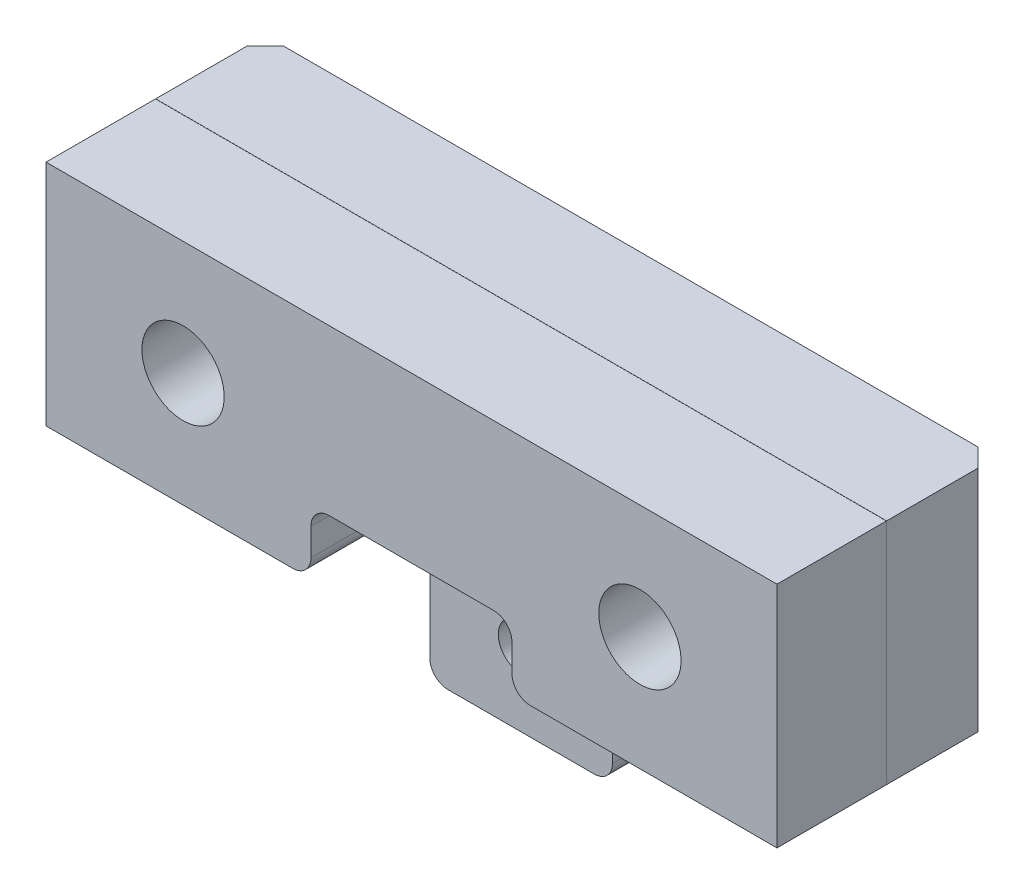
from build123d import *

# Parameters (mm, degrees)
SKETCH1_W                = 80
SKETCH1_H                = 24
BOSS_EXTRUDE1_DEPTH      = 20
CHAMFER1_SIZE            = 2
SKETCH9_W                = 20
SKETCH9_H                = 15
CUT_EXTRUDE1_DEPTH       = 12
M6_TAPPED_HOLE1_D        = 5
M6_TAPPED_HOLE1_DEPTH    = 15
M6_TAPPED_HOLE1_TIP      = 1.502151548
M8_CLEARANCE_HOLE1_D     = 9
M8_CLEARANCE_HOLE1_DEPTH = 30
M8_CLEARANCE_HOLE1_TIP   = 2.703872786
SKETCH16_W               = 30
SKETCH16_H               = 15
CUT_EXTRUDE2_DEPTH       = 86.883642214
FILLET1_R                = 5
FILLET2_R                = 2
SKETCH17_W               = 22
SKETCH17_H               = 7
CUT_EXTRUDE3_DEPTH       = 12
SKETCH18_W               = 80
SKETCH18_H               = 0.02
CUT_EXTRUDE4_DEPTH       = 88.183714076
FILLET3_R                = 2


with BuildPart() as part:
    # Sketch1 → Boss-Extrude1 (new, symmetric)
    with BuildSketch(Plane(origin=(0, 0, 0), x_dir=(1, 0, 0), z_dir=(0, 1, 0))):
        with Locations((40, 12)):
            Rectangle(SKETCH1_W, SKETCH1_H)
    extrude(amount=BOSS_EXTRUDE1_DEPTH, both=True)

    # Chamfer1
    chamfer1_edges = [part.edges().sort_by_distance(p)[0] for p in [
        (0, 0, -24),
        (80, 0, -24),
    ]]
    chamfer(chamfer1_edges, length=CHAMFER1_SIZE)

    # Sketch9 → Cut-Extrude1 (cut)
    with BuildSketch(Plane.XY):
        with Locations((40, -12.5)):
            Rectangle(SKETCH9_W, SKETCH9_H)
    extrude(amount=-CUT_EXTRUDE1_DEPTH, mode=Mode.SUBTRACT)

    # M6 Tapped Hole1
    with Locations(Plane(origin=(0, 0, -24), x_dir=(-1, 0, 0), z_dir=(0, 0, -1))):
        with Locations((-40, -12)):
            Hole(M6_TAPPED_HOLE1_D / 2, depth=M6_TAPPED_HOLE1_DEPTH)
            with Locations((0, 0, -(M6_TAPPED_HOLE1_DEPTH + M6_TAPPED_HOLE1_TIP / 2))):  # 118° drill point
                Cone(0, M6_TAPPED_HOLE1_D / 2, M6_TAPPED_HOLE1_TIP, mode=Mode.SUBTRACT)

    # M8 Clearance Hole1
    with Locations(Plane(origin=(0, 0, -24), x_dir=(-1, 0, 0), z_dir=(0, 0, -1))):
        with Locations((-65, 7.5), (-15, 7.5)):
            Hole(M8_CLEARANCE_HOLE1_D / 2, depth=M8_CLEARANCE_HOLE1_DEPTH)
            with Locations((0, 0, -(M8_CLEARANCE_HOLE1_DEPTH + M8_CLEARANCE_HOLE1_TIP / 2))):  # 118° drill point
                Cone(0, M8_CLEARANCE_HOLE1_D / 2, M8_CLEARANCE_HOLE1_TIP, mode=Mode.SUBTRACT)

    # Sketch16 → Cut-Extrude2 (cut, through all)
    with BuildSketch(Plane(origin=(0, 0, -24), x_dir=(-1, 0, 0), z_dir=(0, 0, -1))):
        with Locations((-65, -12.5)):
            Rectangle(SKETCH16_W, SKETCH16_H)
        with Locations((-15, -12.5)):
            Rectangle(SKETCH16_W, SKETCH16_H)
    extrude(amount=-CUT_EXTRUDE2_DEPTH, mode=Mode.SUBTRACT)

    # Fillet1
    fillet1_edges = [part.edges().sort_by_distance(p)[0] for p in [
        (50, -5, -18),
        (30, -5, -18),
    ]]
    fillet(fillet1_edges, radius=FILLET1_R)

    # Fillet2
    fillet2_edges = [part.edges().sort_by_distance(p)[0] for p in [
        (50, -20, -18),
        (30, -20, -18),
    ]]
    fillet(fillet2_edges, radius=FILLET2_R)

    # Sketch17 → Cut-Extrude3 (cut)
    with BuildSketch(Plane.XY):
        with Locations((40, -1.5)):
            Rectangle(SKETCH17_W, SKETCH17_H)
    extrude(amount=-CUT_EXTRUDE3_DEPTH, mode=Mode.SUBTRACT)

    # Sketch18 → Cut-Extrude4 (cut, through all)
    with BuildSketch(Plane.XZ.offset(5)):
        with Locations((40, -11.99)):
            Rectangle(SKETCH18_W, SKETCH18_H)
    extrude(amount=-CUT_EXTRUDE4_DEPTH, mode=Mode.SUBTRACT)


with BuildPart() as cut_extrude4_piece_1:
    # of the separate pieces the step leaves, piece 1, a body of its own (cut_extrude4_pieces)
    add(part.part.solids().sort_by_distance((50, -18, -24))[0])


with BuildPart() as cut_extrude4_piece_2:
    # of the separate pieces the step leaves, piece 2, a body of its own (cut_extrude4_pieces)
    add(part.part.solids().sort_by_distance((51, -5, -11.98))[0])

    # Fillet3
    fillet3_edges = [cut_extrude4_piece_2.edges().sort_by_distance(p)[0] for p in [
        (51, 2, -5.99),
        (51, -5, -5.99),
        (29, 2, -5.99),
        (29, -5, -5.99),
    ]]
    fillet(fillet3_edges, radius=FILLET3_R)


solid = Compound([cut_extrude4_piece_1.part, cut_extrude4_piece_2.part])
